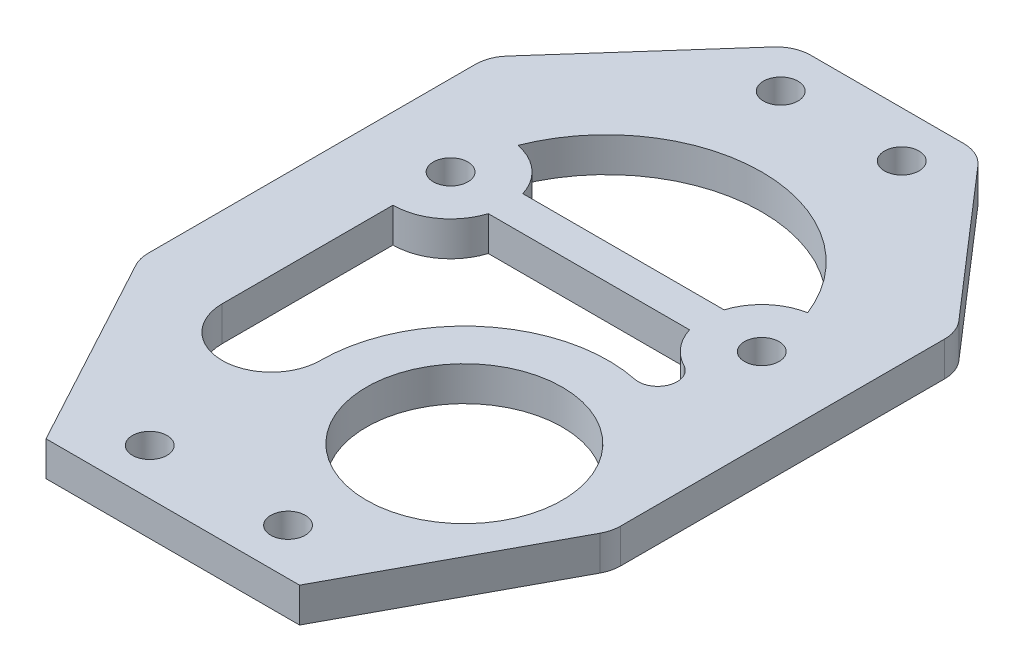
from build123d import *

# Parameters (mm, degrees)
SKETCH1_R           = 8.5
SKETCH1_R_2         = 1.5
BOSS_EXTRUDE1_DEPTH = 3
FILLET1_R           = 3


with BuildPart() as part:
    # Sketch1 → Boss-Extrude1 (new body)
    with BuildSketch(Plane(origin=(0, 0, 0), x_dir=(1, 0, 0), z_dir=(0, 1, 0))):
        Polygon((-11, 0), (11, 0), (20.489621783, 17.605313925), (20.489621783, 47.605313925), (8, 62), (-8, 62), (-20.509243816, 47.910305032), (-20.509243816, 17.610706132), align=None)
        with Locations(Location((7.519679741, 17.780252273, 0), (0, 0, 270))):
            Circle(SKETCH1_R, mode=Mode.SUBTRACT)
        with Locations(Location((6, 4, 0), (0, 0, 270))):
            Circle(SKETCH1_R_2, mode=Mode.SUBTRACT)
        with Locations(Location((-6, 4, 0), (0, 0, 90))):
            Circle(SKETCH1_R_2, mode=Mode.SUBTRACT)
        with Locations(Location((-5.25, 57.999859765, 0), (0, 0, 270))):
            Circle(SKETCH1_R_2, mode=Mode.SUBTRACT)
        with Locations(Location((5.25, 57.999859765, 0), (0, 0, 270))):
            Circle(SKETCH1_R_2, mode=Mode.SUBTRACT)
        with Locations(Location((-13.5, 37.605313925, 0), (0, 0, 270))):
            Circle(SKETCH1_R_2, mode=Mode.SUBTRACT)
        with Locations(Location((13.5, 37.605313925, 0), (0, 0, 270))):
            Circle(SKETCH1_R_2, mode=Mode.SUBTRACT)
        with BuildLine():
            Line((-8.730303993, 39.105313925), (8.730303993, 39.105313925))
            ThreePointArc((8.730303993, 39.105313925), (10.179901517, 41.34388933), (12.574074074, 42.518832133))
            ThreePointArc((12.574074074, 42.518832133), (0, 51.105313925), (-12.574074074, 42.518832133))
            ThreePointArc((-12.574074074, 42.518832133), (-10.179901517, 41.34388933), (-8.730303993, 39.105313925))
        make_face(mode=Mode.SUBTRACT)
        with BuildLine():
            Line((-8.730303993, 36.105313925), (8.730303993, 36.105313925))
            ThreePointArc((8.730303993, 36.105313925), (9.667400631, 34.394210987), (11.187975781, 33.171969363))
            ThreePointArc((11.187975781, 33.171969363), (11.998189223, 31.105465162), (10.062695821, 30.018841621))
            ThreePointArc((10.062695821, 30.018841621), (-0.366780245, 27.478383479), (-4.980318958, 17.785955551))
            ThreePointArc((-4.980318958, 17.785955551), (-9.241131059, 13.528058523), (-13.5, 17.787899155))
            Line((-13.5, 17.787899155), (-13.5, 32.605313925))
            ThreePointArc((-13.5, 32.605313925), (-10.541960108, 33.574185051), (-8.730303993, 36.105313925))
        make_face(mode=Mode.SUBTRACT)
    extrude(amount=BOSS_EXTRUDE1_DEPTH)

    # Fillet1
    fillet1_edges = [part.edges().sort_by_distance(p)[0] for p in [
        (-20.509243816, 1.5, -17.610706132),
        (-20.509243816, 1.5, -47.910305032),
        (-8, 1.5, -62),
        (8, 1.5, -62),
        (20.489621783, 1.5, -47.605313925),
        (20.489621783, 1.5, -17.605313925),
    ]]
    fillet(fillet1_edges, radius=FILLET1_R)


solid = part.part
